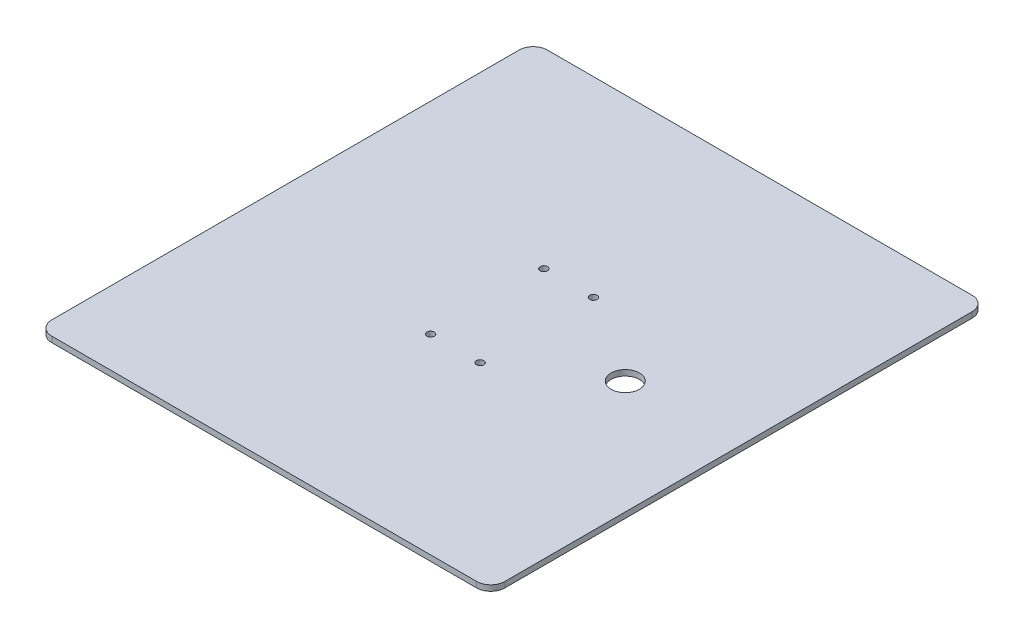
SolidWorks part; units mm, degrees
ref_plane "Front Plane" through (0, 0, 0) normal (0, 0, 1) x (1, 0, 0)
ref_plane "Top Plane" through (0, 0, 0) normal (0, 1, 0) x (1, 0, 0)
ref_plane "Right Plane" through (0, 0, 0) normal (1, 0, 0) x (0, 0, -1)
sketch "Sketch1" plane through (0, 0, 0) normal (0, 1, 0) x (1, 0, 0)
  line L1 (160, -175) -> (-160, -175)
  line L2 (160, -175) -> (160, 175)
  line L3 (160, 175) -> (-160, 175)
  line L4 (-160, -175) -> (-160, 175)
  line L5 (160, -175) -> (-160, 175) construction
  line L6 (160, 175) -> (-160, -175) construction
  point P0 (0, 0)
  dimension "D1" = 320
  dimension "D2" = 350
extrude "Boss-Extrude1" add sketch "Sketch1" along normal blind 4
hole_wizard "Ø5.2 (5.2) Diameter Hole1" positions "Sketch2" profile "Sketch3" hole size "Ø5.2" standard "GB"
sketch "Sketch2" plane through (0, 4, 0) normal (0, 1, 0) x (1, 0, 0)
  line L1 (-17.5, 40) -> (17.5, 40) construction
  line L2 (-17.5, 40) -> (-17.5, -40) construction
  line L3 (-17.5, -40) -> (17.5, -40) construction
  line L4 (17.5, 40) -> (17.5, -40) construction
  line L6 (0, 0) -> (0, 40) construction
  line L8 (-17.5, 0) -> (0, 0) construction
  point P0 (-17.5, 40)
  point P4 (17.5, -40)
  point P91 (-17.5, -40)
  point P92 (17.5, 40)
  dimension "D1" = 35
  dimension "D2" = 80
sketch "Sketch3" plane through (-17.5, 4, -40) normal (1, 0, 0) x (0, 0, 1)
  line L0 (0, 0) -> (0, 11.6622)
  line L1 (0, 11.6622) -> (2.6, 10.1)
  line L2 (2.6, 10.1) -> (2.6, 0)
  line L5 (2.6, 0) -> (0, 0)
  line L10 (0, 11.6622) -> (-2.6, 10.1) construction
  line L11 (0, -6.35) -> (0, 107.95) construction
  dimension "孔直径" = 5.2
  dimension "孔深度" = 10.1
  dimension "导头角度" = 118
fillet "Fillet1" radius 10 4 edges at (-160, 2, 175) (160, 2, 175) (160, 2, -175) (-160, 2, -175)
sketch "Sketch4" plane through (0, 4, 0) normal (0, 1, 0) x (1, 0, 0)
  line L0 (160, -165) -> (160, 165) construction
  line L1 (0, 0) -> (80, 0) construction
  circle A0 centre (80, 0) radius 10
  dimension "D1" = 20
  dimension "D2" = 80
extrude "Cut-Extrude1" cut sketch "Sketch4" against normal through all
